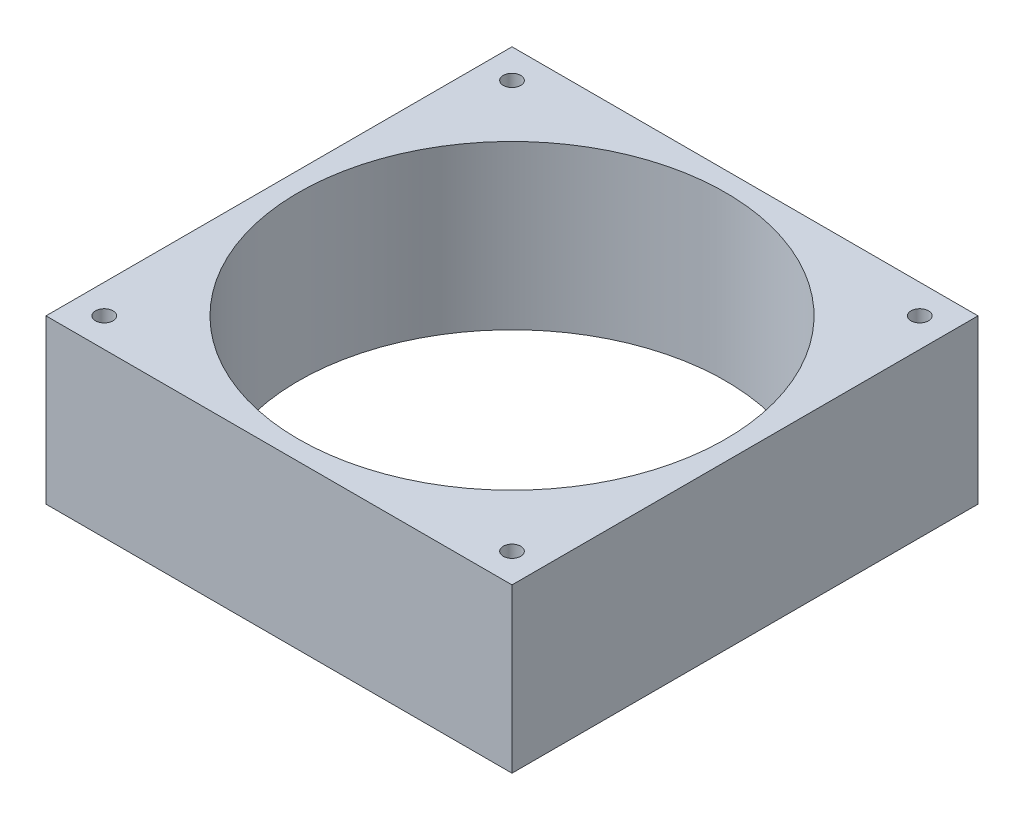
SolidWorks part; units mm, degrees
material "橡胶"
ref_plane "前视基准面" through (0, 0, 0) normal (0, 0, 1) x (1, 0, 0)
ref_plane "上视基准面" through (0, 0, 0) normal (0, 1, 0) x (1, 0, 0)
ref_plane "右视基准面" through (0, 0, 0) normal (1, 0, 0) x (0, 0, -1)
sketch "草图1" plane through (0, 0, 0) normal (0, 1, 0) x (1, 0, 0)
  line L1 (-60, 60) -> (60, 60)
  line L2 (-60, 60) -> (-60, -60)
  line L3 (-60, -60) -> (60, -60)
  line L4 (60, 60) -> (60, -60)
  line L5 (-60, 60) -> (60, -60) construction
  line L6 (-60, -60) -> (60, 60) construction
  point P0 (0, 0)
  dimension "D1" = 120
  dimension "D2" = 120
extrude "凸台-拉伸1" add sketch "草图1" along normal mid plane 42
sketch "草图2" plane through (0, 21, 0) normal (0, 1, 0) x (1, 0, 0)
  line L0 (0, 0) -> (44.308, 0) construction
  line L1 (0, 0) -> (0, 93.5595) construction
  circle A0 centre (0, 0) radius 55
  circle A1 centre (-52.5, 52.5) radius 2.25
  circle A2 centre (52.5, 52.5) radius 2.25
  circle A3 centre (52.5, -52.5) radius 2.25
  circle A4 centre (-52.5, -52.5) radius 2.25
  dimension "D1" = 110
  dimension "D2" = 4.5
  dimension "D3" = 105
  dimension "D4" = 105
extrude "切除-拉伸1" cut sketch "草图2" against normal through all both and the other way through all
